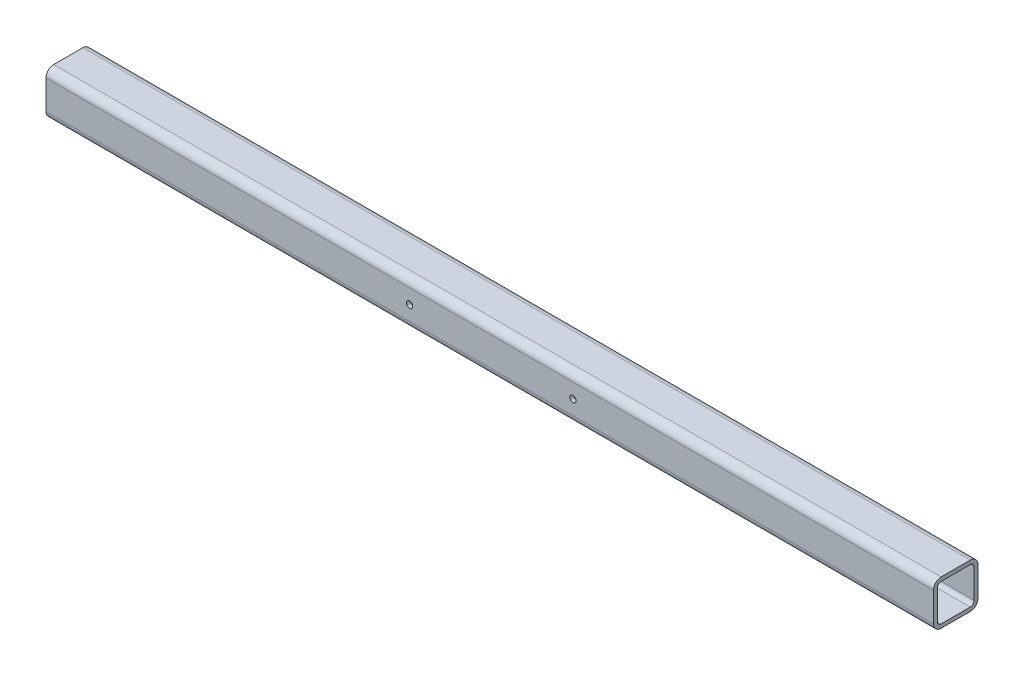
SolidWorks part; units mm, degrees
ref_plane "前视基准面" through (0, 0, 0) normal (0, 0, 1) x (1, 0, 0)
ref_plane "上视基准面" through (0, 0, 0) normal (0, 1, 0) x (1, 0, 0)
ref_plane "右视基准面" through (0, 0, 0) normal (1, 0, 0) x (0, 0, -1)
sketch3d "3D草图1"
  line L0 (0, 0, 0) -> (598, 0, 0)
  dimension "D1" = 598
other "结构构件1"
ref_plane "基准面1" through (0, 0, 0) normal (1, 0, 0) x (0, 0, -1)
sketch "Sketch1" plane through (0, 0, 0) normal (1, 0, 0) x (0, 0, -1)
  line L0 (-9.8, -12.4) -> (9.8, -12.4)
  line L1 (-12.4, -9.8) -> (-12.4, 9.8)
  line L2 (9.8, 12.4) -> (-9.8, 12.4)
  line L3 (12.4, 9.8) -> (12.4, -9.8)
  line L4 (-9.8, -15) -> (9.8, -15)
  line L5 (-15, -9.8) -> (-15, 9.8)
  line L6 (9.8, 15) -> (-9.8, 15)
  line L7 (15, 9.8) -> (15, -9.8)
  arc A0 (15, 9.8) -> (9.8, 15) centre (9.8, 9.8) ccw
  arc A1 (9.8, -15) -> (15, -9.8) centre (9.8, -9.8) ccw
  arc A2 (-15, -9.8) -> (-9.8, -15) centre (-9.8, -9.8) ccw
  arc A3 (-9.8, 15) -> (-15, 9.8) centre (-9.8, 9.8) ccw
  arc A4 (-9.8, 12.4) -> (-12.4, 9.8) centre (-9.8, 9.8) ccw
  arc A5 (12.4, 9.8) -> (9.8, 12.4) centre (9.8, 9.8) ccw
  arc A6 (9.8, -12.4) -> (12.4, -9.8) centre (9.8, -9.8) ccw
  arc A7 (-12.4, -9.8) -> (-9.8, -12.4) centre (-9.8, -9.8) ccw
  point P0 (-15, 0)
  point P1 (15, 0)
  point P2 (0, 15)
  point P3 (0, -15)
  point P4 (0, 0)
  point P5 (-15, -15)
  point P6 (15, -15)
  point P7 (15, 15)
  point P8 (-15, 15)
  point P33 (0, 0)
  dimension "D1" = 5.2
  dimension "Thickness" = 2.6
  dimension "V_leg" = 30
hole_wizard "M5 螺纹孔1" positions "草图4" profile "草图3" tap size "M5" standard "Iso" end condition through all
sketch "草图4" plane through (0, 0, 15) normal (0, 0, 1) x (1, 0, 0)
  point P0 (355, 0)
  point P3 (245, 0)
sketch "草图3" plane through (355, 0, 15) normal (1, 0, 0) x (0, -1, 0)
  line L0 (0, 0) -> (0, 30)
  line L1 (0, 30) -> (2.1, 30)
  line L2 (2.1, 30) -> (2.1, 0)
  line L5 (2.1, 0) -> (0, 0)
  line L11 (0, -6.35) -> (0, 107.95) construction
  dimension "通孔螺纹孔钻头直径" = 4.2
  dimension "通孔螺纹孔钻头深度" = 30
cosmetic thread "孔螺蚊线1"
cosmetic thread "孔螺蚊线2"
